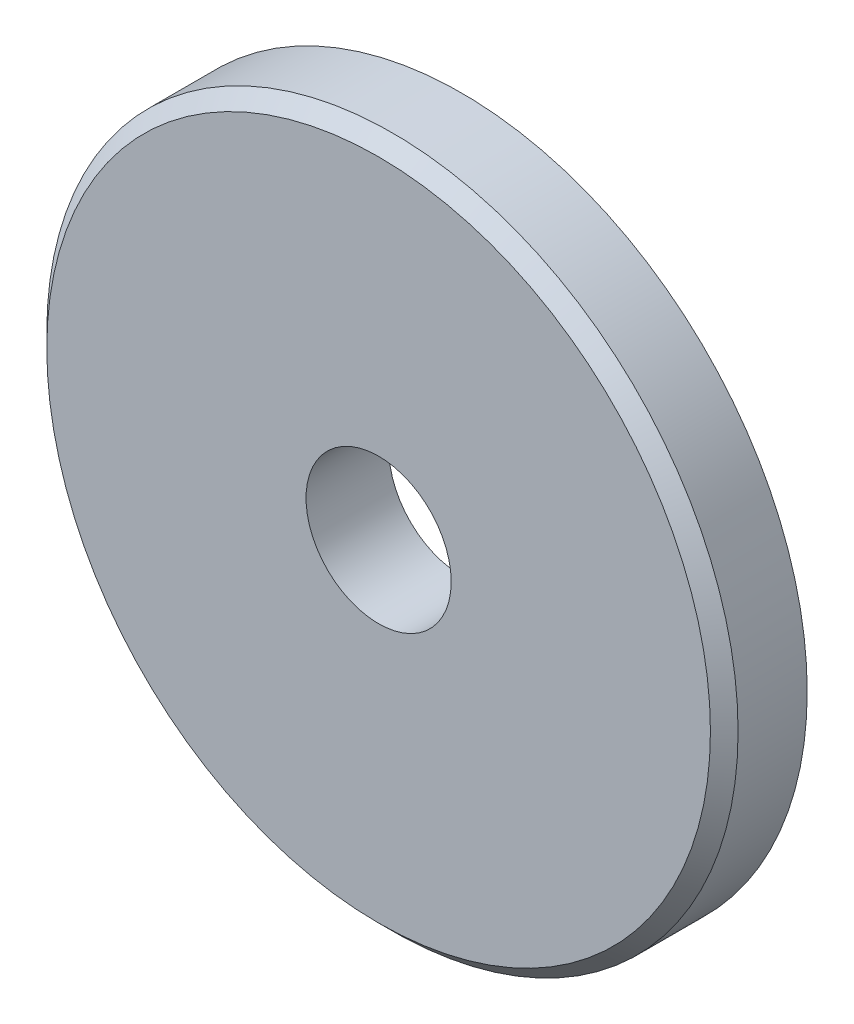
SolidWorks part; units mm, degrees
ref_plane "前视基准面" through (0, 0, 0) normal (0, 0, 1) x (1, 0, 0)
ref_plane "上视基准面" through (0, 0, 0) normal (0, 1, 0) x (1, 0, 0)
ref_plane "右视基准面" through (0, 0, 0) normal (1, 0, 0) x (0, 0, -1)
sketch "草图1" plane through (0, 0, 0) normal (0, 0, 1) x (1, 0, 0)
  circle A0 centre (0, 0) radius 25
  circle A1 centre (0, 0) radius 5.25
  dimension "D1" = 50
  dimension "D2" = 10.5
extrude "凸台-拉伸1" add sketch "草图1" along normal blind 6
chamfer "倒角1" distance 1 angle 45 1 edges at (25, 0, 6)
